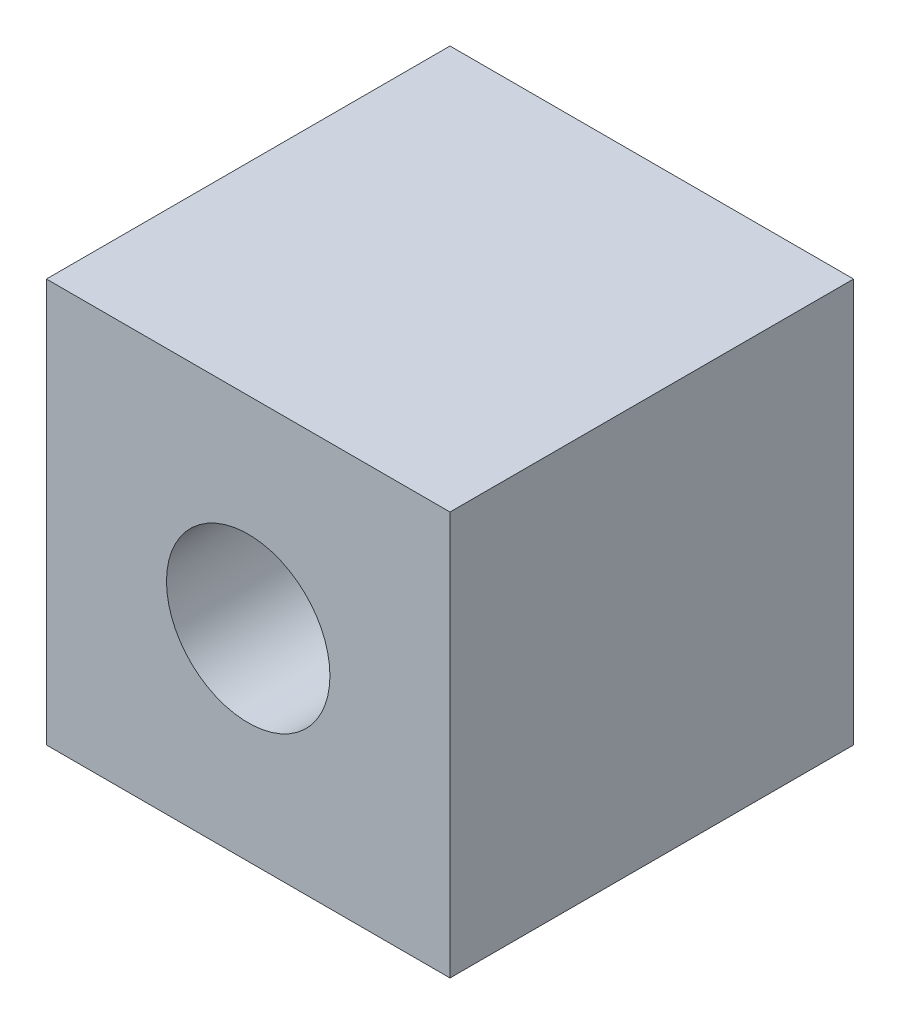
SolidWorks part; units mm, degrees
ref_plane "前视基准面" through (0, 0, 0) normal (0, 0, 1) x (1, 0, 0)
ref_plane "上视基准面" through (0, 0, 0) normal (0, 1, 0) x (1, 0, 0)
ref_plane "右视基准面" through (0, 0, 0) normal (1, 0, 0) x (0, 0, -1)
other "Configuration Table"
sketch "草图1" plane through (0, 0, 0) normal (0, 0, 1) x (1, 0, 0)
  line L0 (-20, -20) -> (20, -20)
  line L1 (20, -20) -> (20, 20)
  line L2 (20, 20) -> (-20, 20)
  line L3 (-20, 20) -> (-20, -20)
  point P0 (0, 0)
  dimension "D1" = 20
  dimension "D2" = 40
  dimension "D3" = 20
  dimension "D4" = 40
extrude "凸台-拉伸1" add sketch "草图1" against normal mid plane 40
sketch "草图2" plane through (0, 0, 0) normal (0, 0, 1) x (1, 0, 0)
  circle A0 centre (0, 0) radius 8.1
  point P0 (0, 0)
  dimension "D1" = 16.2
extrude "切除-拉伸1" cut sketch "草图2" against normal mid plane 80
